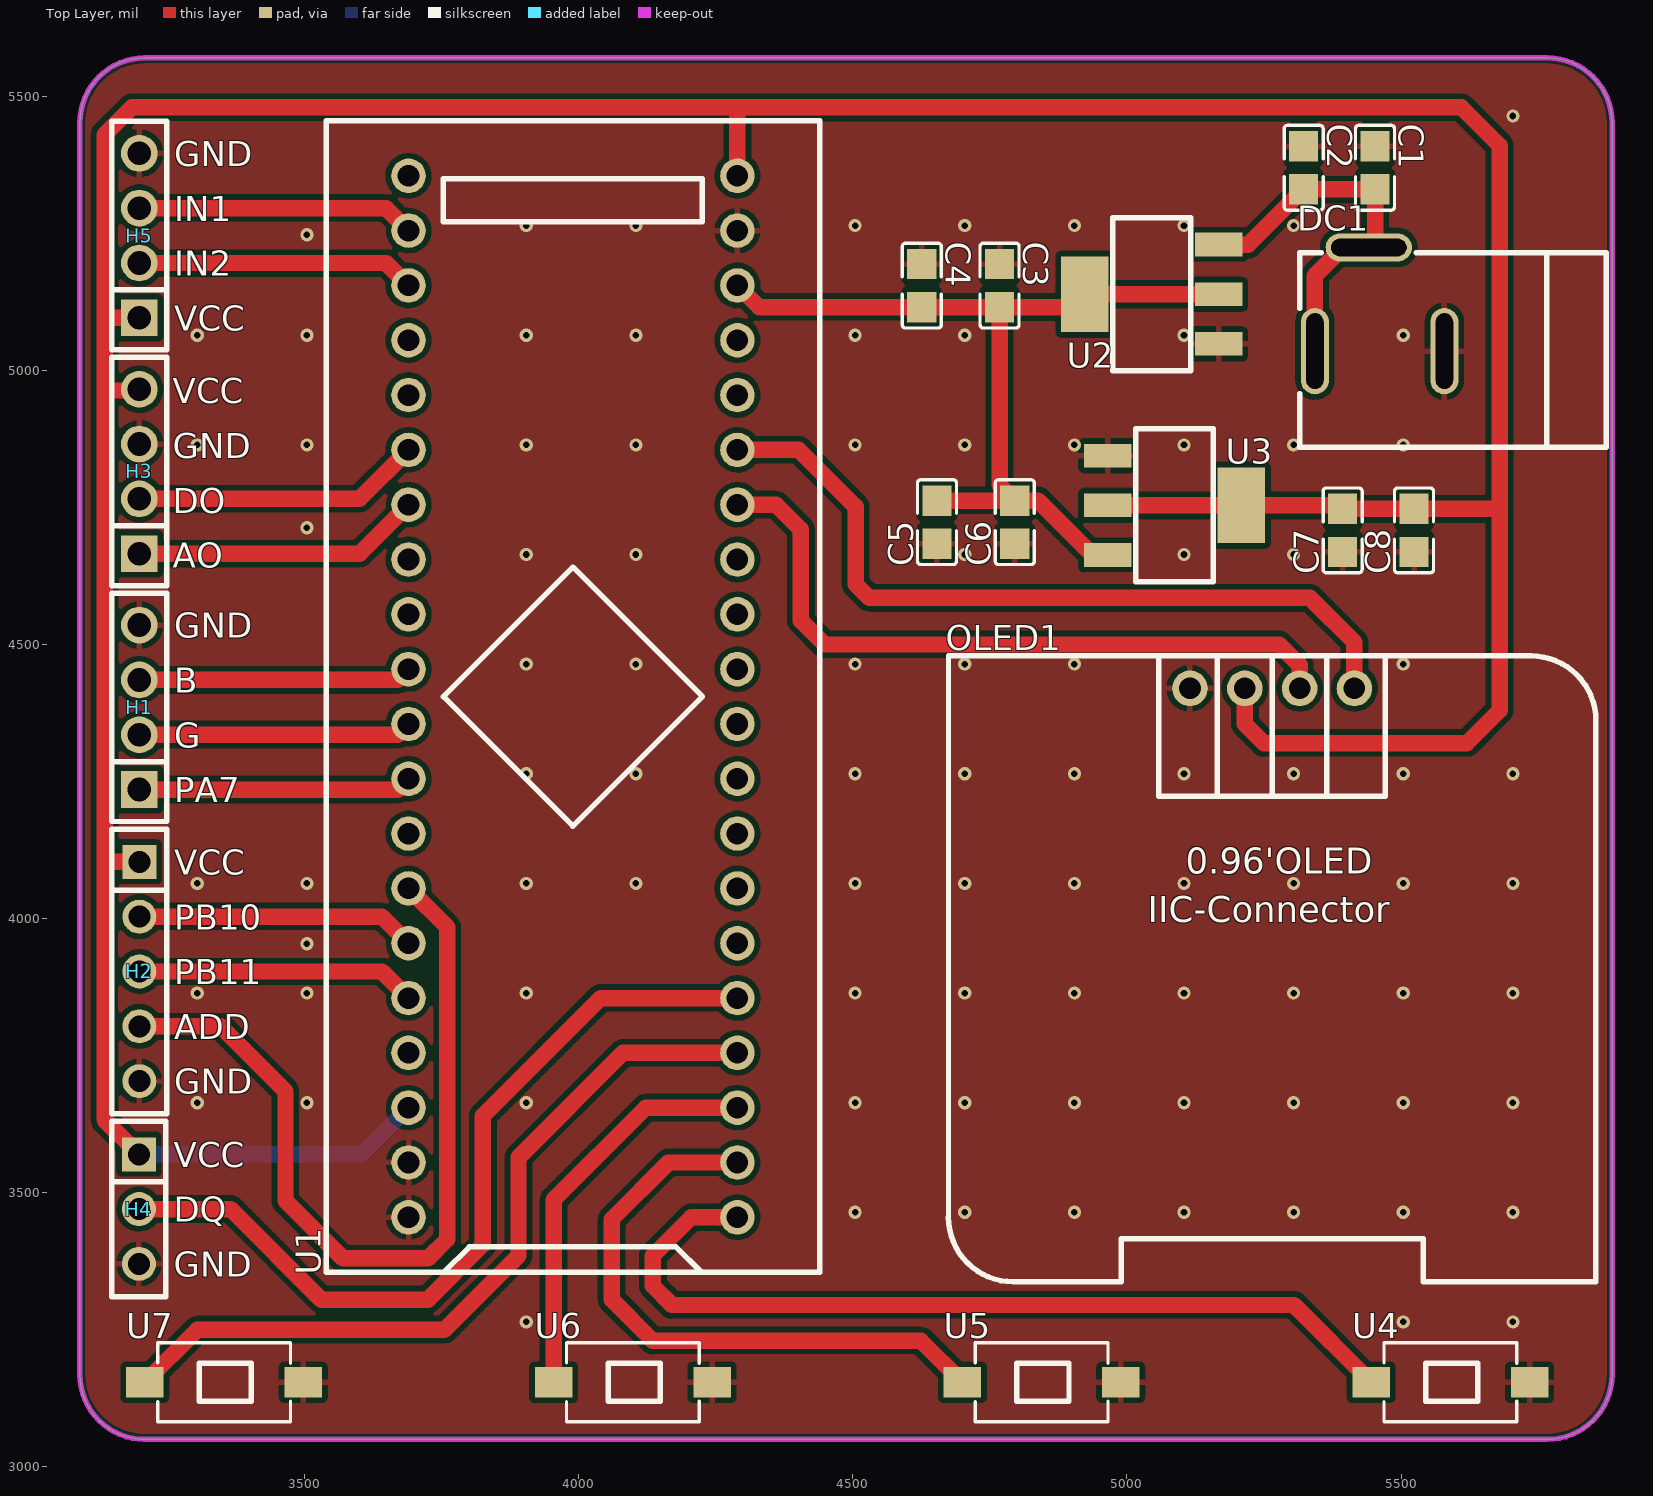
[diagram p0: Top Layer view]
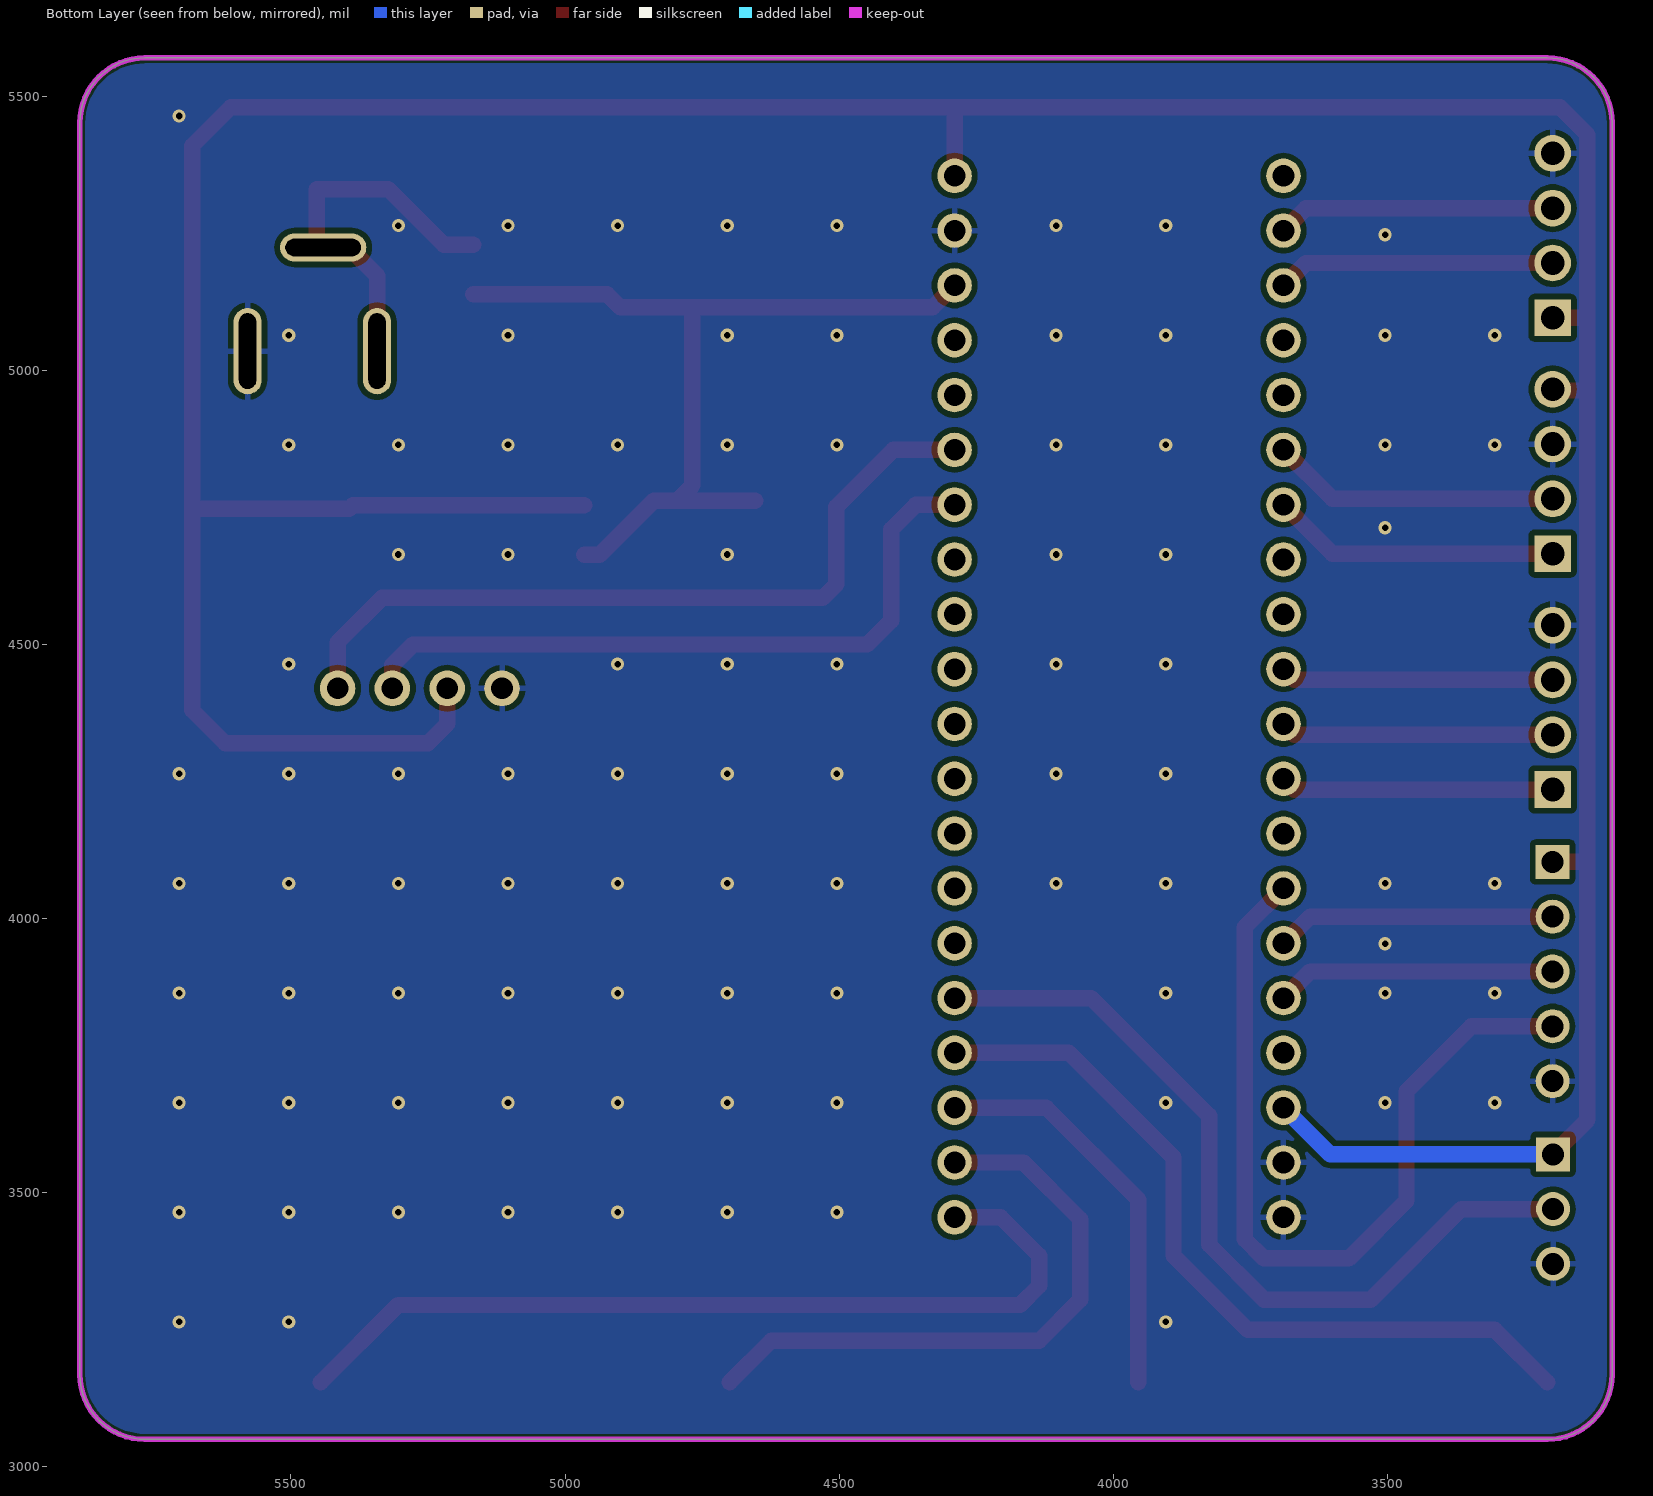
[diagram p1: Bottom Layer view, seen from below]
# Altium PCB MISC51501.pcbdoc
Units mil, origin at the board's own origin, x right, y up, seen from the top; angles counter-clockwise.
Board outline 2795 x 2520 mil, 2 copper layers (Top Layer, Bottom Layer), stack 62.206 mil thick; 22 components, 38 nets, 99 pads, 90 vias.

## Layer stack, top to bottom
Top Solder Mask Layer: solder mask 0.394, Dk 3.3
Top Layer: signal copper 1.379
Dielectric1: surface 59.449, FR4, Dk 4.5
Bottom Layer: signal copper 1.378
Bottom Solder Mask Layer: solder mask 0.394, Dk 3.3

## Board outline
3208.11,5570 ccw(c3208.11,5451.89) 3090,5451.89 3090,3168.11 ccw(c3208.11,3168.11) 3208.11,3050 5766.89,3050 ccw(c5766.89,3168.11) 5885,3168.11 5885,5451.89 ccw(c5766.89,5451.89) 5766.89,5570

## Design rules (kind name [scope] priority, off if disabled: settings)
BoardOutlineClearance copperThickness2oz_1 [All] p2 off: genericclearance=7.99 ignorepadtopadclearanceinfootprint=FALSE except(0: Arc-SplitContinuation Track-SplitContinuation SMDPad-SplitContinuation THPad-SplitContinuation Via-SplitContinuation Fill-SplitContinuation Region-SplitContinuation Poly-SplitContinuation Text-SplitContinuation Hole-SplitContinuation; 5.98: Arc-CutoutEdge Track-CutoutEdge SMDPad-CutoutEdge THPad-CutoutEdge Via-CutoutEdge Text-CutoutEdge; 6.9: Hole-OutlineEdge Hole-CutoutEdge; 10: Poly-OutlineEdge Poly-CutoutEdge; 11.81: Arc-OutlineEdge Track-OutlineEdge SMDPad-OutlineEdge THPad-OutlineEdge Via-OutlineEdge Fill-OutlineEdge Region-OutlineEdge Text-OutlineEdge Fill-CutoutEdge Region-CutoutEdge)
BoardOutlineClearance Plane_innerPlane_1 [All] p4 off: genericclearance=4.02 ignorepadtopadclearanceinfootprint=FALSE except(0: Arc-SplitContinuation Track-SplitContinuation SMDPad-SplitContinuation THPad-SplitContinuation Via-SplitContinuation Fill-SplitContinuation Region-SplitContinuation Poly-SplitContinuation Text-SplitContinuation Hole-SplitContinuation; 5.98: Arc-CutoutEdge Track-CutoutEdge SMDPad-CutoutEdge THPad-CutoutEdge Via-CutoutEdge Text-CutoutEdge; 6.9: Hole-OutlineEdge Hole-CutoutEdge; 10: Poly-OutlineEdge Poly-CutoutEdge; 11.81: Arc-OutlineEdge Track-OutlineEdge SMDPad-OutlineEdge THPad-OutlineEdge Via-OutlineEdge Fill-OutlineEdge Region-OutlineEdge Text-OutlineEdge Fill-CutoutEdge Region-CutoutEdge)
BoardOutlineClearance Copper_copperRegion_1 [All] p6 off: genericclearance=4.02 ignorepadtopadclearanceinfootprint=FALSE except(0: Arc-SplitContinuation Track-SplitContinuation SMDPad-SplitContinuation THPad-SplitContinuation Via-SplitContinuation Fill-SplitContinuation Region-SplitContinuation Poly-SplitContinuation Text-SplitContinuation Hole-SplitContinuation; 5.98: Arc-CutoutEdge Track-CutoutEdge SMDPad-CutoutEdge THPad-CutoutEdge Via-CutoutEdge Text-CutoutEdge; 6.9: Hole-OutlineEdge Hole-CutoutEdge; 10: Poly-OutlineEdge Poly-CutoutEdge; 11.81: Arc-OutlineEdge Track-OutlineEdge SMDPad-OutlineEdge THPad-OutlineEdge Via-OutlineEdge Fill-OutlineEdge Region-OutlineEdge Text-OutlineEdge Fill-CutoutEdge Region-CutoutEdge)
BoardOutlineClearance copperThickness1oz_1 [All] p8: genericclearance=4.02 ignorepadtopadclearanceinfootprint=FALSE except(0: Arc-SplitContinuation Track-SplitContinuation SMDPad-SplitContinuation THPad-SplitContinuation Via-SplitContinuation Fill-SplitContinuation Region-SplitContinuation Poly-SplitContinuation Text-SplitContinuation Hole-SplitContinuation; 5.98: Arc-CutoutEdge Track-CutoutEdge SMDPad-CutoutEdge THPad-CutoutEdge Via-CutoutEdge Text-CutoutEdge; 6.9: Hole-OutlineEdge Hole-CutoutEdge; 10: Poly-OutlineEdge Poly-CutoutEdge; 11.81: Arc-OutlineEdge Track-OutlineEdge SMDPad-OutlineEdge THPad-OutlineEdge Via-OutlineEdge Fill-OutlineEdge Region-OutlineEdge Text-OutlineEdge Fill-CutoutEdge Region-CutoutEdge)
Clearance copperThickness2oz [All] p1 off: gap=7.99 ignorepadtopadclearanceinfootprint=FALSE except(5.98: SMDPad-Track SMDPad-SMDPad THPad-Track SMDPad-THPad THPad-THPad Track-Via SMDPad-Via THPad-Via Via-Via Fill-SMDPad Region-SMDPad Fill-THPad Region-THPad Fill-Via Region-Via Fill-Fill Fill-Region Region-Region Arc-Track Arc-SMDPad Arc-THPad Arc-Via Fill-Arc Region-Arc Arc-Arc Text-Track SMDPad-Text Text-THPad Text-Via Fill-Text Region-Text Arc-Text Text-Text; 6.9: Hole-Track Hole-SMDPad Hole-THPad Hole-Via Fill-Hole Region-Hole Hole-Arc Hole-Text; 10: Poly-Track Poly-SMDPad Poly-THPad Poly-Via Poly-Fill Poly-Region Poly-Poly Poly-Arc Poly-Text Poly-Hole; 11.81: Fill-Track Region-Track)
Clearance Plane_innerPlane [All] p3 off: gap=4.02 ignorepadtopadclearanceinfootprint=FALSE except(5.98: SMDPad-Track SMDPad-SMDPad THPad-Track SMDPad-THPad THPad-THPad Track-Via SMDPad-Via THPad-Via Via-Via Fill-SMDPad Region-SMDPad Fill-THPad Region-THPad Fill-Via Region-Via Fill-Fill Fill-Region Region-Region Arc-Track Arc-SMDPad Arc-THPad Arc-Via Fill-Arc Region-Arc Arc-Arc Text-Track SMDPad-Text Text-THPad Text-Via Fill-Text Region-Text Arc-Text Text-Text; 6.9: Hole-Track Hole-SMDPad Hole-THPad Hole-Via Fill-Hole Region-Hole Hole-Arc Hole-Text; 10: Poly-Track Poly-SMDPad Poly-THPad Poly-Via Poly-Fill Poly-Region Poly-Poly Poly-Arc Poly-Text Poly-Hole; 11.81: Fill-Track Region-Track)
Clearance Copper_copperRegion [All] p5 off: gap=4.02 ignorepadtopadclearanceinfootprint=FALSE except(5.98: SMDPad-Track SMDPad-SMDPad THPad-Track SMDPad-THPad THPad-THPad Track-Via SMDPad-Via THPad-Via Via-Via Fill-SMDPad Region-SMDPad Fill-THPad Region-THPad Fill-Via Region-Via Fill-Fill Fill-Region Region-Region Arc-Track Arc-SMDPad Arc-THPad Arc-Via Fill-Arc Region-Arc Arc-Arc Text-Track SMDPad-Text Text-THPad Text-Via Fill-Text Region-Text Arc-Text Text-Text; 6.9: Hole-Track Hole-SMDPad Hole-THPad Hole-Via Fill-Hole Region-Hole Hole-Arc Hole-Text; 10: Poly-Track Poly-SMDPad Poly-THPad Poly-Via Poly-Fill Poly-Region Poly-Poly Poly-Arc Poly-Text Poly-Hole; 11.81: Fill-Track Region-Track)
Clearance copperThickness1oz [All] p7: gap=4.02 ignorepadtopadclearanceinfootprint=FALSE except(5.98: SMDPad-Track SMDPad-SMDPad THPad-Track SMDPad-THPad THPad-THPad Track-Via SMDPad-Via THPad-Via Via-Via Fill-SMDPad Region-SMDPad Fill-THPad Region-THPad Fill-Via Region-Via Fill-Fill Fill-Region Region-Region Arc-Track Arc-SMDPad Arc-THPad Arc-Via Fill-Arc Region-Arc Arc-Arc Text-Track SMDPad-Text Text-THPad Text-Via Fill-Text Region-Text Arc-Text Text-Text; 6.9: Hole-Track Hole-SMDPad Hole-THPad Hole-Via Fill-Hole Region-Hole Hole-Arc Hole-Text; 10: Poly-Track Poly-SMDPad Poly-THPad Poly-Via Poly-Fill Poly-Region Poly-Poly Poly-Arc Poly-Text Poly-Hole; 11.81: Fill-Track Region-Track)
DiffPairsRouting differentialPair [All] p1: maxlimit=6 minlimit=6 mostfreqgap=6 toplayer_minwidth=5 toplayer_prefwidth=10 toplayer_maxwidth=100 toplayer_mingap=6 toplayer_prefgap=6 toplayer_maxgap=6 bottomlayer_minwidth=5 bottomlayer_prefwidth=10 bottomlayer_maxwidth=100 bottomlayer_mingap=6 bottomlayer_prefgap=6 bottomlayer_maxgap=6 maxuncoupledlength=10
HoleToHoleClearance otherClearance [All] p1: gap=11.81 allowstackedmicrovias=TRUE
Length netLength [All] p1: minlimit=0 maxlimit=0
PasteMaskExpansion pasteMaskExpansion [All] p1: expansion=0
PlaneConnect innerPlane [All] p1: planeconnectstyle=Relief reliefexpansion=20 reliefentries=4 reliefconductorwidth=10 reliefairgap=10
PolygonConnect copperRegion [All] p1: connectstyle=Relief reliefconductorwidth=10 reliefentries=4 polygonreliefangle="90 Angle" airgapwidth=10 via.connectstyle=Relief via.reliefconductorwidth=10 via.reliefentries=4 via.polygonreliefangle="90 Angle" via.airgapwidth=10
RoutingVias viaSize [All] p1: holewidth=12.01 width=24.02 viastyle="Through Hole" minholewidth=11.81 minwidth=19.68 maxholewidth=248.03 maxwidth=393.7
SolderMaskExpansion solderMaskExpansion [IsVia] p1: expansion=-1000 istentingtop=TRUE
SolderMaskExpansion solderMaskExpansion [All] p2: expansion=2 istentingtop=FALSE
Width copperThickness2oz_2 [All] p1 off: maxlimit=100 minlimit=8 preferedwidth=10
Width copperThickness1oz_2 [All] p2: maxlimit=100 minlimit=5 preferedwidth=10

## Components (designator, comment, footprint, x,y, rotation, side; value= is the part's Value field where it differs from the comment)
C1 "10uF" C0805 5452.61,5369.7 r270 top
C2 "100nF" C0805 5322.31,5369.7 r270 top
C3 "10uF" C0805 4767.68,5154.7 r270 top
C4 "100nF" C0805 4625.72,5154.7 r270 top
C5 "10uF" C0805 4653.44,4723.14 r90 top
C6 "100nF" C0805 4795.4,4723.14 r90 top
C7 "10uF" C0805 5393.45,4708.14 r90 top
C8 "100nF" C0805 5523.75,4708.14 r90 top
DC1 "" DC-2.0 5466,5024.7 r0 top
H1 "" HDR-TH_4P-P2.54-V-F 3198.39,4385.34 r90 top
H2 "" HDR-TH_5P-P2.54-V-F 3198.39,3903.46 r270 top
H3 "" HDR-TH_4P-P2.54-V-F 3198.39,4815.65 r90 top
H4 "" HDR-TH_3P-P2.54-V-F 3197.6,3470 r270 top
H5 "" HDR-TH_4P-P2.54-V-F 3198.39,5245.96 r90 top
OLED1 "" 0.96OLED_4P 5265,4420 r0 top
U1 "STM32F103C8T6-Card" CONN-TH_L53.3-W22.9_STM32F103C8T6-CARD 3989.4,4405 r90 top
U2 "AMS1117-5.0" SOT_223 5044.26,5138.92 r90 top
U3 "AMS1117-3.3" SOT_223 5087.93,4753.92 r270 top
U4 "BX-TS-26-365TP" KEY-SMD_L6.0-W3.5-LS8.0-1 5590,3154.19 r0 top
U5 "BX-TS-26-365TP" KEY-SMD_L6.0-W3.5-LS8.0-1 4844.3,3154.19 r0 top
U6 "BX-TS-26-365TP" KEY-SMD_L6.0-W3.5-LS8.0-1 4098.6,3154.19 r0 top
U7 "BX-TS-26-365TP" KEY-SMD_L6.0-W3.5-LS8.0-1 3352.91,3154.19 r0 top

## Footprints (in the part's own frame and the unit in brackets; to place one, negate y for a bottom-side part, rotate by r counter-clockwise, add the part's x,y. Pads: shape width x height; smd on the part's side, far side on the other; paste and mask are expansions set on the pad)
0.96OLED_4P [mm]
  round 1.65 hole 1 copper offset 0,0: 1(-3.81,-0.001) 2(-1.27,0.002) 3(1.27,0.002) 4(3.81,0.002)
  silkscreen extent -15,-27.5 15,1.5
C0805 [mm]
  rect 1.41x1.35 smd paste-100 mask+0.051: 1(-1,0) 2(1,0)
  silkscreen extent -1.96,-0.9 1.96,0.9
CONN-TH_L53.3-W22.9_STM32F103C8T6-CARD [mm]
  round 1.6 hole 1: 1(-24.13,-7.62) 2(-21.59,-7.62) 3(-19.05,-7.62) 4(-16.51,-7.62) 5(-13.97,-7.62) 6(-11.43,-7.62) 7(-8.89,-7.62) 8(-6.35,-7.62) 9(-3.81,-7.62) 10(-1.27,-7.62) 11(1.27,-7.62) 12(3.81,-7.62) 13(6.35,-7.62) 14(8.89,-7.62) 15(11.43,-7.62) 16(13.97,-7.62) 17(16.51,-7.62) 18(19.05,-7.62) 19(21.59,-7.62) 20(24.13,-7.62) 21(24.13,7.62) 22(21.59,7.62) 23(19.05,7.62) 24(16.51,7.62) 25(13.97,7.62) 26(11.43,7.62) 27(8.89,7.62) 28(6.35,7.62) 29(3.81,7.62) 30(1.27,7.62) 31(-1.27,7.62) 32(-3.81,7.62) 33(-6.35,7.62) 34(-8.89,7.62) 35(-11.43,7.62) 36(-13.97,7.62) 37(-16.51,7.62) 38(-19.05,7.62) 39(-21.59,7.62) 40(-24.13,7.62)
  silkscreen extent -26.67,-11.43 26.67,11.43
DC-2.0 [mil]
  oval 157.5x51.2 hole 31.5 slot 137.8 at 0 deg paste+0 mask+2: 2(-24.7,199.5)
  oval 51.2x157.5 hole 31.5 slot 137.8 at 90 deg paste+0 mask+2: 3(113.1,10.5) 4(-123.1,10.5)
  silkscreen extent -151,-165 408,190
HDR-TH_3P-P2.54-V-F [mil]
  rect 62x62 hole 40.16: 1(-100,0)
  round 62 hole 40.16: 2(0,0) 3(100,0)
  silkscreen extent -160,-49 160,49
HDR-TH_4P-P2.54-V-F [mm]
  rect 1.7x1.7 hole 1.1: 1(-3.81,0)
  round 1.7 hole 1.1: 2(-1.27,0) 3(1.27,0) 4(3.81,0)
  silkscreen extent -5.29,-1.27 5.29,1.27
HDR-TH_5P-P2.54-V-F [mil]
  rect 62x62 hole 40.16: 1(-200,0)
  round 62 hole 40.16: 2(-100,0) 3(0,0) 4(100,0) 5(200,0)
  silkscreen extent -260,-50 260,50
KEY-SMD_L6.0-W3.5-LS8.0-1 [mm]
  rect 1.74x1.4 smd: 1(-3.67,0) 2(3.67,0)
  silkscreen extent -3.08,-1.83 3.08,1.83
SOT_223 [mil]
  rect 43.3x86.6 smd paste+0 mask+2: 1(-90.5,-123.05) 2(0,-123.05) 3(90.6,-123.05)
  rect 137.8x86.6 smd paste+0 mask+2: 4(0,120.95)
  silkscreen extent -140,-72 140,70

## Via types
v1: diameter 24.02, hole 12, Top Layer to Bottom Layer, 90 vias

## Nets (pads, with @x,y where several pads share a name; then routed paths per layer and width w, separated by ;. In a path a pad name is that pad's centre, name@x,y a point inside that pad or via, vN(x,y) a via of type N, cw(c..) or ccw(c..) an arc to the next point about the centre after c; other vN are vias at no path point)
5V: C3.2 C4.2 C5.2 C6.2 U1.18 U2.2 U2.4 U3.3 | length 1620.9
  Top Layer w30: U1.18 4329.07,5115.33 C4.2 C3.2 ; C5.2 C6.2 ; U3.3 4937.02,4663.32 4837.83,4762.51 C6.2 ; U2.2 U2.4 4899.73,5115.33 C3.2 ; C3.2 4767.68,4790.23 C6.2
12V: C1.2 C2.2 DC1.2 DC1.4 U2.3 | length 695.2
  Top Layer w30: U2.3 5221.5,5229.52 C2.2 C1.2 5452.61,5235.51 DC1.2 5394.2,5224.2 5342.9,5172.9 DC1.4
ADD: H2.4 U1.34 | length 1537.9
  Top Layer w30: H2.4 3346.54,3803.46 3465,3685 3465,3485 3570,3380 3725,3380 3760,3415 3760,3984.4 U1.34
AO: H3.1 U1.27 | length 528
  Top Layer w30: H3.1 3600.05,4665.65 U1.27
B: H1.3 U1.30 | length 499.2
  Top Layer w30: H1.3 3669.74,4435.34 U1.30
DO: H3.2 U1.26 | length 528
  Top Layer w30: H3.2 3600.05,4765.65 U1.26
DQ: H4.2 U1.5 | length 1525.6
  Top Layer w30: H4.2 3365,3470 3530,3305 3725,3305 3825,3405 3825,3640 4040,3855 U1.5
G: H1.2 U1.31 | length 499.2
  Top Layer w30: H1.2 3669.74,4335.34 U1.31
GND: C1.1 C2.1 C3.1 C4.1 C5.1 C6.1 C7.1 C8.1 DC1.3 H1.4 H2.5 H3.3 H4.3 H5.4 OLED1.1 U1.19 U1.39 U1.40 U2.1 U3.1 U4.2 U5.2 U6.2 U7.2
  other v1: 3904.1,3264.1 5504.1,3264.1 5704.1,3264.1 4504.1,3464.1 4704.1,3464.1 4904.1,3464.1 5104.1,3464.1 5304.1,3464.1 5504.1,3464.1 5704.1,3464.1 3304.1,3664.1 3504.1,3664.1 3904.1,3664.1 4504.1,3664.1 4704.1,3664.1 4904.1,3664.1 5104.1,3664.1 5304.1,3664.1 5504.1,3664.1 5704.1,3664.1 3304.1,3864.1 3504.1,3864.1 3904.1,3864.1 4504.1,3864.1 4704.1,3864.1 4904.1,3864.1 5104.1,3864.1 5304.1,3864.1 5504.1,3864.1 5704.1,3864.1 3504.1,3954.16 3304.1,4064.1 3504.1,4064.1 3904.1,4064.1 4104.1,4064.1 4504.1,4064.1 4704.1,4064.1 4904.1,4064.1 5104.1,4064.1 5304.1,4064.1 5504.1,4064.1 5704.1,4064.1 3904.1,4264.1 4104.1,4264.1 4504.1,4264.1 4704.1,4264.1 4904.1,4264.1 5104.1,4264.1 5304.1,4264.1 5504.1,4264.1 5704.1,4264.1 3904.1,4464.1 4104.1,4464.1 4504.1,4464.1 4704.1,4464.1 4904.1,4464.1 5504.1,4464.1 3904.1,4664.1 4104.1,4664.1 4704.1,4664.1 5104.1,4664.1 5304.1,4664.1 3504.1,4712.9 3304.1,4864.1 3504.1,4864.1 3904.1,4864.1 4104.1,4864.1 4504.1,4864.1 4704.1,4864.1 4904.1,4864.1 5104.1,4864.1 5304.1,4864.1 5504.1,4864.1 3304.1,5064.1 3504.1,5064.1 3904.1,5064.1 4104.1,5064.1 4504.1,5064.1 4704.1,5064.1 5104.1,5064.1 5504.1,5064.1 3504.1,5247.6 3904.1,5264.1 4104.1,5264.1 4504.1,5264.1 4704.1,5264.1 4904.1,5264.1 5104.1,5264.1 5304.1,5264.1 5704.1,5464.1
IN1: H5.3 U1.22 | length 508
  Top Layer w30: H5.3 3648.44,5295.96 U1.22
IN2: H5.2 U1.23 | length 508
  Top Layer w30: H5.2 3648.44,5195.96 U1.23
K1: U1.1 U4.1 | length 1621.7
  Top Layer w30: U1.1 4205,3455 4135,3385 4135,3330 4170,3295 5304.7,3295 U4.1
K2: U1.2 U5.1 | length 1121
  Top Layer w30: U1.2 4163.58,3555 4060,3451.42 4060,3305 4135,3230 4624,3230 U5.1
K3: U1.3 U6.1 | length 737.7
  Top Layer w30: U6.1 3954.11,3486.96 4122.16,3655 U1.3
K4: U1.4 U7.1 | length 1434.9
  Top Layer w30: U7.1 3304.23,3250 3755,3250 3890,3385 3890,3564.26 4080.74,3755 U1.4
NRST: U1.37
OLEDSCL: OLED1.3 U1.14 | length 1286.7
  Top Layer w30: U1.14 4360,4755 4405,4710 4405,4543.58 4448.58,4500 5277.53,4500 5315,4462.53 OLED1.3@5315,4420.05
OLEDSDA: OLED1.4 U1.15 | length 1437.8
  Top Layer w30: U1.15 4401.42,4855 4505,4751.42 4505,4610 4530,4585 5333.95,4585 5415,4503.95 OLED1.4@5415,4420.05
PA0: U1.25
PA3: U1.28
PA4: U1.29
PA7: H1.1 U1.32 | length 499.2
  Top Layer w30: H1.1 3669.74,4235.34 U1.32
PA9: U1.6
PA10: U1.7
PA11: U1.8
PA12: U1.9
PA15: U1.10
PB0: U1.33
PB3: U1.11
PB4: U1.12
PB5: U1.13
PB8: U1.16
PB9: U1.17
PB10: H2.2 U1.35 | length 511.1
  Top Layer w30: H2.2 3640.94,4003.46 U1.35
PB11: H2.3 U1.36 | length 511.1
  Top Layer w30: H2.3 3640.94,3903.46 U1.36
PC15: U1.24
VBAT: U1.21
VCC: C7.2 C8.2 H2.1 H3.4 H4.1 H5.1 OLED1.2 U1.20 U1.38 U3.2 U3.4 | length 7641
  Top Layer w30: H4.1 3135,3632.6 3135,4103.46 ; H2.1 3135,4103.46 ; H3.4 3196.04,4963.31 3135,4963.31 ; H5.1 3135,5095.96 ; U1.20 4289.4,5480 ; U3.2 U3.4 5387.04,4753.92 C7.2 C8.2 5680,4747.51 ; OLED1.2@5215,4420.05 5215,4355 5250,4320 5620,4320 5680,4380 5680,4747.51 ; 3135,4103.46 3135,4963.31 ; 3135,4963.31 3135,5095.96 ; 3135,5095.96 3135,5430 3185,5480 4289.4,5480 ; 4289.4,5480 5610,5480 5680,5410 5680,4747.51
  Bottom Layer w30: H4.1 3604.39,3570 U1.38

## Polygon pours and split planes (outlines as drawn)
GND on Top Layer (solid, remove dead copper, pour order 0): 3020,5655 3020,3015 5970,3015 5970,5655
GND on Bottom Layer (solid, remove dead copper, pour order 2): 3000,5680 3000,3000 5965,3000 5965,5680

## Keep-outs
Board Outline Layer:
  the board outline again, w10

## Silkscreen, mask and mechanical layers (free items; w line width, h text height)
Top Silkscreen Layer:
  text "GND" at 3261.75,5372.5 h45
  text "IN1" at 3261.75,5272.5 h45
  text "IN2" at 3261.75,5172.5 h45
  text "VCC" at 3261.75,5072.5 h45
  text "VCC" at 3259.41,4939.85 h45
  text "GND" at 3259.41,4839.85 h45
  text "DO" at 3259.41,4739.85 h45
  text "AO" at 3259.41,4639.85 h45
  text "GND" at 3261.75,4511.88 h45
  text "B" at 3261.75,4411.88 h45
  text "G" at 3261.75,4311.88 h45
  text "PA7" at 3261.75,4211.88 h45
  text "VCC" at 3261.75,4080 h45
  text "PB10" at 3261.75,3980 h45
  text "PB11" at 3261.75,3880 h45
  text "ADD" at 3261.75,3780 h45
  text "GND" at 3261.75,3680 h45
  text "VCC" at 3260.96,3546.54 h45
  text "DQ" at 3260.96,3446.54 h45
  text "GND" at 3260.96,3346.54 h45